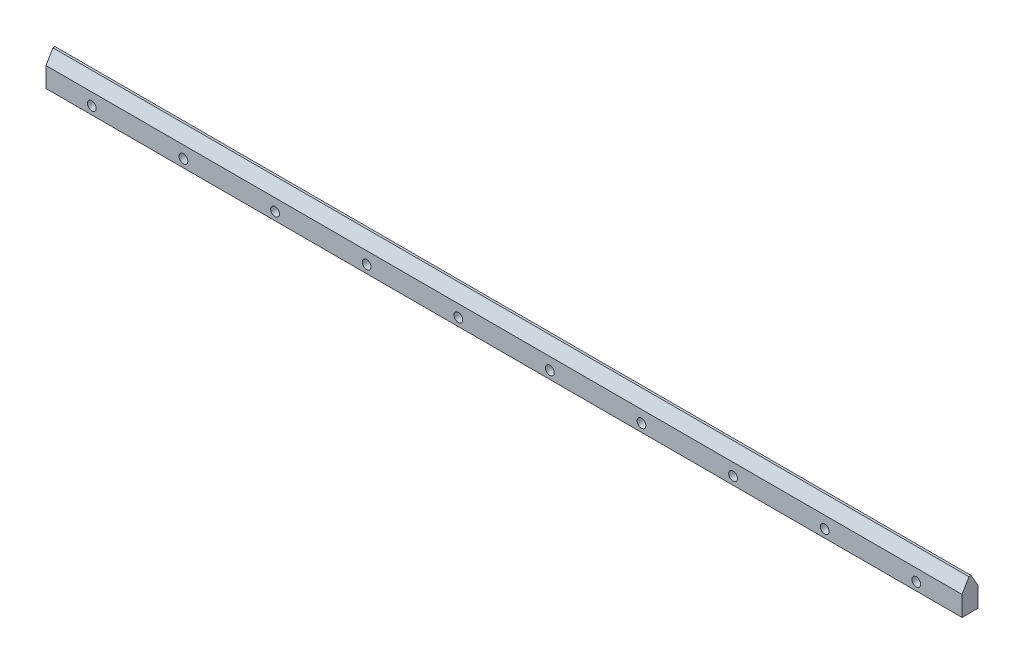
from build123d import *

# Parameters (mm, degrees)
BOSS_EXTRUDE1_DEPTH = 2300
SKETCH2_R           = 5
CUT_EXTRUDE1_DEPTH  = 2301.695547003
SKETCH3_R           = 11
CUT_EXTRUDE2_DEPTH  = 20
LPATTERN1_COUNT     = 10
LPATTERN1_PITCH     = 230


with BuildPart() as part:
    # Sketch1 → Boss-Extrude1 (new body)
    with BuildSketch(Plane(origin=(0, 0, 0), x_dir=(0, 0, -1), z_dir=(1, 0, 0))):
        Polygon((-2.679491924, 40), (-20, 10), (-20, -40), (20, -40), (20, 10), (2.679491924, 40), align=None)
    extrude(amount=BOSS_EXTRUDE1_DEPTH)

    # Sketch2 → Cut-Extrude1 (cut, through all)
    with BuildSketch(Plane.XY.offset(20)):
        with Locations((115, -20)):
            Circle(SKETCH2_R)
    cut_extrude1 = extrude(amount=-CUT_EXTRUDE1_DEPTH, mode=Mode.SUBTRACT)

    # Sketch3 → Cut-Extrude2 (cut)
    with BuildSketch(Plane.XY.offset(20)):
        with Locations((115, -20)):
            Circle(SKETCH3_R)
    cut_extrude2 = extrude(amount=-CUT_EXTRUDE2_DEPTH, mode=Mode.SUBTRACT)

    # LPattern1: Cut-Extrude1, Cut-Extrude2 ×10
    with Locations(*[(i * LPATTERN1_PITCH, 0, 0) for i in range(1, LPATTERN1_COUNT)]):
        add(cut_extrude1, mode=Mode.SUBTRACT)
        add(cut_extrude2, mode=Mode.SUBTRACT)


solid = part.part
